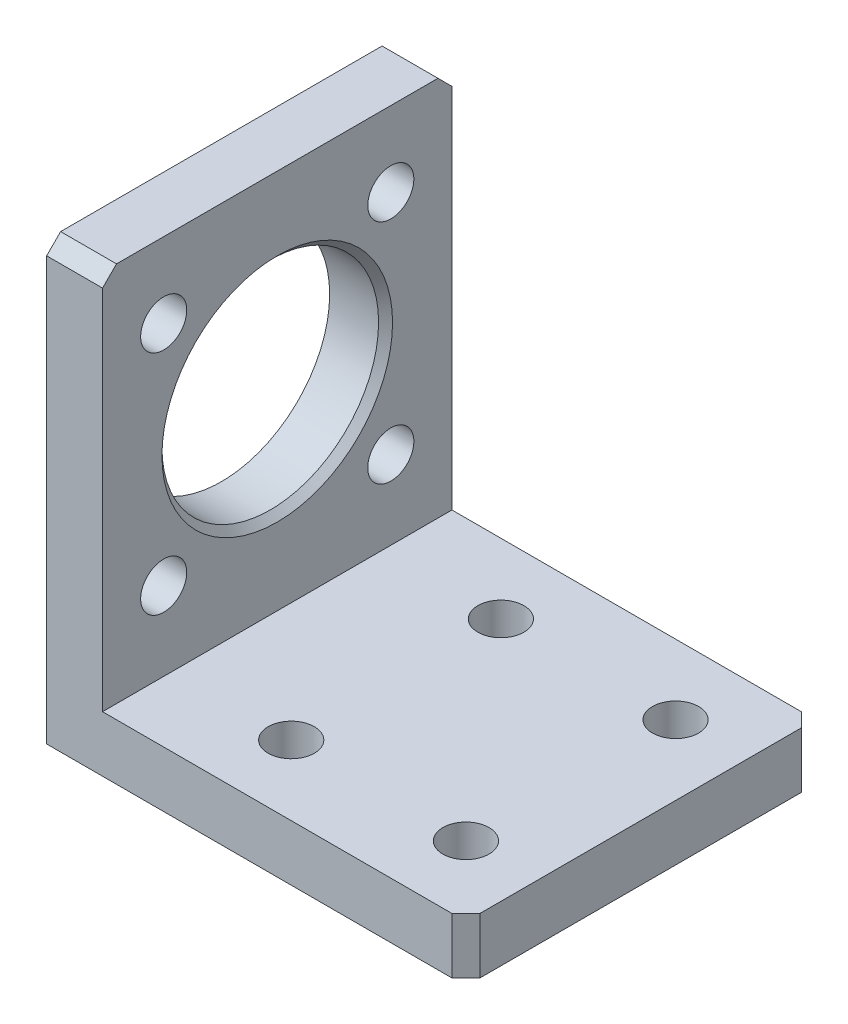
SolidWorks part; units mm, degrees
material "Q235-A"
ref_plane "Front Plane" through (0, 0, 0) normal (0, 0, 1) x (1, 0, 0)
ref_plane "Top Plane" through (0, 0, 0) normal (0, 1, 0) x (1, 0, 0)
ref_plane "Right Plane" through (0, 0, 0) normal (1, 0, 0) x (0, 0, -1)
sketch "Sketch1" plane through (0, 0, 0) normal (0, 0, 1) x (1, 0, 0)
  line L0 (-40.8198, 34.9062) -> (-40.8198, -27.5937)
  line L1 (-40.8198, -27.5937) -> (19.1802, -27.5937)
  line L2 (19.1802, -27.5937) -> (19.1802, -19.5938)
  line L3 (19.1802, -19.5938) -> (-32.8198, -19.5938)
  line L4 (-32.8198, -19.5938) -> (-32.8198, 34.9062)
  line L5 (-32.8198, 34.9062) -> (-40.8198, 34.9062)
  dimension "D1" = 60
  dimension "D2" = 8
  dimension "D3" = 62.5
  dimension "D4" = 8
extrude "Boss-Extrude1" add sketch "Sketch1" along normal blind 50
sketch "Sketch2" plane through (-32.8198, 0, 0) normal (1, 0, 0) x (0, 0, -1)
  line L0 (-50, -27.5937) -> (0, -27.5937) construction
  line L1 (-50, 34.9062) -> (0, 34.9062) construction
  line L3 (-41.25, -8.3437) -> (-8.75, -8.3437)
  line L4 (-41.25, -8.3437) -> (-41.25, 24.1563)
  line L5 (-41.25, 24.1563) -> (-8.75, 24.1563)
  line L6 (-8.75, -8.3437) -> (-8.75, 24.1563)
  line L7 (-41.25, -8.3437) -> (-8.75, 24.1563) construction
  line L8 (-41.25, 24.1563) -> (-8.75, -8.3437) construction
  circle A0 centre (-25, 7.9062) radius 10.9771
  point P7 (-25, 34.9062)
  dimension "D1" = 35.5
  dimension "D2" = 0
  dimension "D3" = 32.5
  dimension "D4" = 32.5
hole_wizard "Hole1" positions "Sketch3" profile "Sketch4" legacy end condition through all
sketch "Sketch3" plane through (-32.8198, 0, 0) normal (1, 0, 0) x (0, 0, -1)
  point P0 (-41.25, 24.1563)
  point P3 (-8.75, 24.1563)
  point P6 (-8.75, -8.3437)
  point P9 (-41.25, -8.3437)
sketch "Sketch4" plane through (-32.8198, 24.1563, 41.25) normal (0, 1, 0) x (0, 0, -1)
  line L0 (0, 0) -> (0, 8)
  line L1 (0, 8) -> (3.3, 8)
  line L2 (3.3, 8) -> (3.3, 0)
  line L3 (3.3, 0) -> (0, 0)
  line L4 (0, 110) -> (0, -10) construction
  dimension "直径" = 6.6
  dimension "深度" = 8
hole_wizard "Hole2" positions "Sketch5" profile "Sketch6" legacy end condition through all
sketch "Sketch5" plane through (-32.8198, 0, 0) normal (1, 0, 0) x (0, 0, -1)
  point P0 (-25, 7.9062)
sketch "Sketch6" plane through (-32.8198, 7.9062, 25) normal (0, 1, 0) x (0, 0, -1)
  line L0 (0, 0) -> (0, 8)
  line L1 (0, 8) -> (15.5, 8)
  line L2 (15.5, 8) -> (15.5, 0)
  line L3 (15.5, 0) -> (0, 0)
  line L4 (0, 110) -> (0, -10) construction
  dimension "直径" = 31
  dimension "深度" = 8
chamfer "Chamfer1" distance 1 angle 45 1 edges at (-32.8198, 7.9062, 9.5)
chamfer "Chamfer2" distance 2 angle 45 4 edges at (19.1802, -23.5938, 0) (19.1802, -23.5938, 50) (-36.8198, 34.9062, 0) (-36.8198, 34.9062, 50)
sketch "Sketch7" plane through (0, -19.5938, 0) normal (0, 1, 0) x (1, 0, 0)
  line L0 (-40.8198, -48) -> (-40.8198, -2) construction
  line L1 (-15.8198, -40) -> (9.1802, -40)
  line L2 (-15.8198, -40) -> (-15.8198, -10)
  line L3 (-15.8198, -10) -> (9.1802, -10)
  line L4 (9.1802, -40) -> (9.1802, -10)
  line L5 (19.1802, -48) -> (19.1802, -2) construction
  point P6 (9.1802, -25)
  point P9 (19.1802, -25)
  dimension "D1" = 25
  dimension "D2" = 30
  dimension "D3" = 25
  dimension "D4" = 0
hole_wizard "Hole3" positions "Sketch8" profile "Sketch9" legacy end condition through all
sketch "Sketch8" plane through (0, -19.5938, 0) normal (0, 1, 0) x (1, 0, 0)
  point P0 (-15.8198, -40)
  point P3 (-15.8198, -10)
  point P6 (9.1802, -10)
  point P9 (9.1802, -40)
sketch "Sketch9" plane through (-15.8198, -19.5938, 40) normal (1, 0, 0) x (0, 0, 1)
  line L0 (0, 0) -> (0, 8)
  line L1 (0, 8) -> (3.3, 8)
  line L2 (3.3, 8) -> (3.3, 0)
  line L3 (3.3, 0) -> (0, 0)
  line L4 (0, 110) -> (0, -10) construction
  dimension "直径" = 6.6
  dimension "深度" = 8
